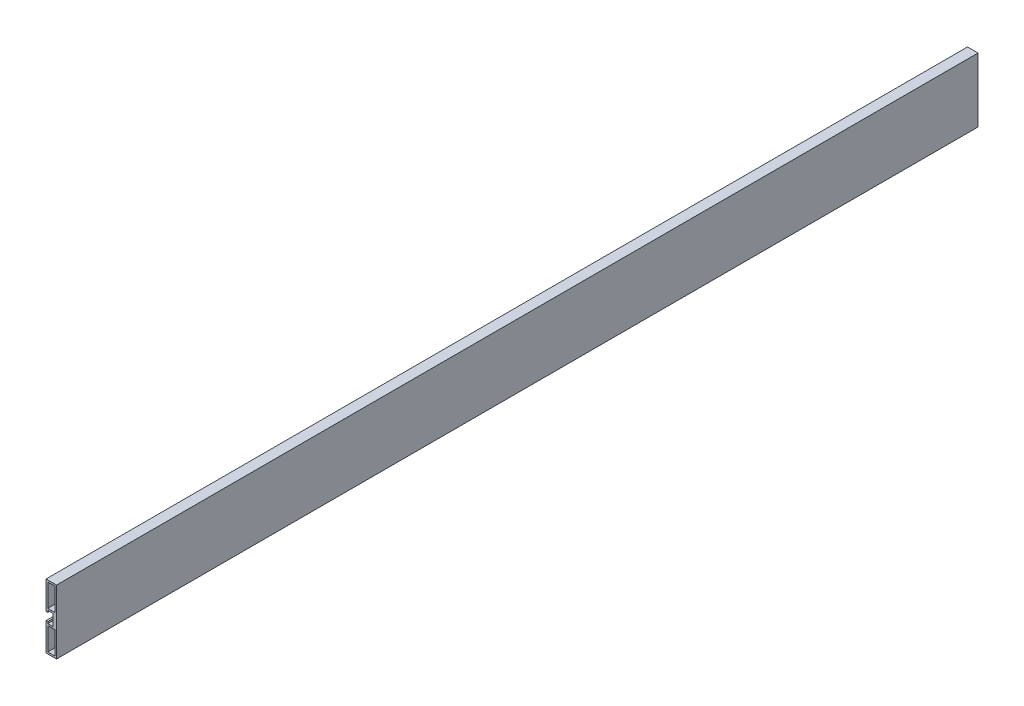
from build123d import *

# Parameters (mm, degrees)
SKETCH_1_W      = 8
SKETCH_1_H      = 26
EXTRUDE_1_DEPTH = 525


with BuildPart() as part:
    # 草图1 → 凸台-拉伸1 (new, symmetric)
    with BuildSketch(Plane.XY):
        Polygon((-12, 4.5), (-10, 4.5), (-10, 6.5), (-4, 6.5), (-4, -6.5), (-10, -6.5), (-10, -4.5), (-12, -4.5), (-12, -36.5), (0, -36.5), (0, 36.5), (-12, 36.5), align=None)
        with Locations((-6, -21.5)):
            Rectangle(SKETCH_1_W, SKETCH_1_H, mode=Mode.SUBTRACT)
        with Locations((-6, 21.5)):
            Rectangle(SKETCH_1_W, SKETCH_1_H, mode=Mode.SUBTRACT)
    extrude(amount=EXTRUDE_1_DEPTH, both=True)


solid = part.part
